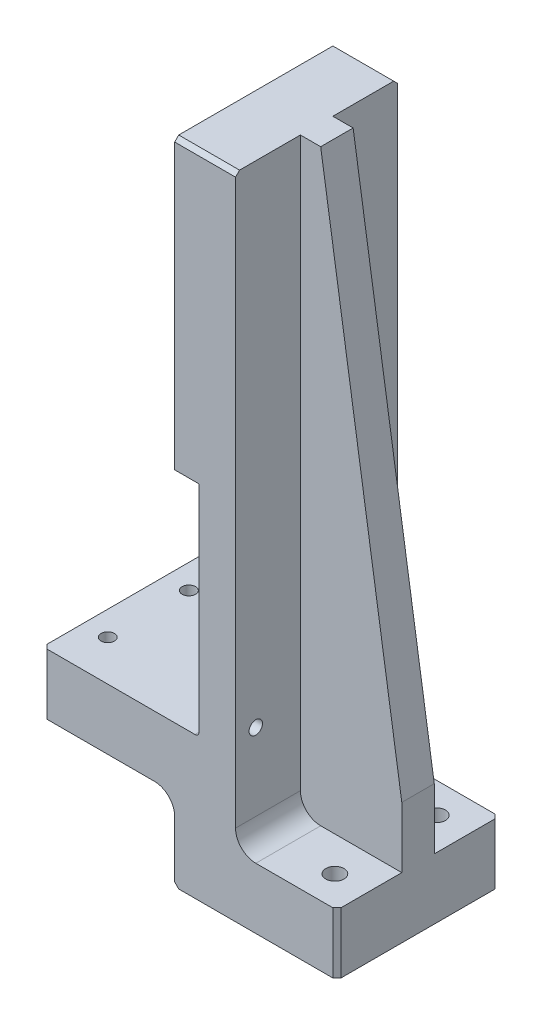
from build123d import *

# Parameters (mm, degrees)
BOSS_EXTRUDE1_DEPTH   = 20
BOSS_EXTRUDE2_DEPTH   = 4
SKETCH3_R             = 2.25
CUT_EXTRUDE2_DEPTH    = 164.343962239
M4_TAPPED_HOLE1_D     = 3.3
M4_TAPPED_HOLE2_D     = 3.3
M4_TAPPED_HOLE2_DEPTH = 11.5
M4_TAPPED_HOLE2_TIP   = 0.991420021
CUT_EXTRUDE3_REACH    = 151.937
SKETCH12_W            = 6
SKETCH12_H            = 54
M4_TAPPED_HOLE3_D     = 3.3
M4_TAPPED_HOLE3_DEPTH = 11.5
M4_TAPPED_HOLE3_TIP   = 0.991420021
CHAMFER1_SIZE         = 1
FILLET1_R             = 1
FILLET2_R             = 5


with BuildPart() as part:
    # Sketch1 → Boss-Extrude1 (new, symmetric)
    with BuildSketch(Plane.XY):
        Polygon((0, 0), (32.5, 0), (32.5, 125), (47.5, 125), (47.5, -20), (72.5, -20), (72.5, -35), (32.5, -35), (32.5, -15), (0, -15), align=None)
    extrude(amount=BOSS_EXTRUDE1_DEPTH, both=True)

    # Sketch2 → Boss-Extrude2 (add, symmetric)
    with BuildSketch(Plane.XY):
        Polygon((47.5, 125), (52.5, 125), (72.5, -5), (72.5, -20), (47.5, -20), align=None)
    extrude(amount=BOSS_EXTRUDE2_DEPTH, both=True)

    # Sketch3 → Cut-Extrude2 (cut, through all)
    with BuildSketch(Plane(origin=(0, -20, 0), x_dir=(1, 0, 0), z_dir=(0, 1, 0))):
        with Locations(Location((64.5, -12.5, 0), (0, 0, 270))):
            Circle(SKETCH3_R)
        with Locations(Location((64.5, 12.5, 0), (0, 0, 270))):
            Circle(SKETCH3_R)
    extrude(amount=-CUT_EXTRUDE2_DEPTH, mode=Mode.SUBTRACT)

    # M4 Tapped Hole1 (through all)
    with Locations(Plane(origin=(0, 0, 0), x_dir=(-1, 0, 0), z_dir=(0, 1, 0))):
        with Locations((-6, -10), (-6, 10)):
            Hole(M4_TAPPED_HOLE1_D / 2)

    # M4 Tapped Hole2
    with Locations(Plane(origin=(32.5, -167.050225356, 16.087508651), x_dir=(0, 0, 1), z_dir=(-1, 0, 0))):
        with Locations((-16.087508651, 276.050225356), (-16.087508651, 251.050225356)):
            Hole(M4_TAPPED_HOLE2_D / 2, depth=M4_TAPPED_HOLE2_DEPTH)
            with Locations((0, 0, -(M4_TAPPED_HOLE2_DEPTH + M4_TAPPED_HOLE2_TIP / 2))):  # 118° drill point
                Cone(0, M4_TAPPED_HOLE2_D / 2, M4_TAPPED_HOLE2_TIP, mode=Mode.SUBTRACT)

    # Sketch12 → Cut-Extrude3 (cut, up to next)
    with BuildSketch(Plane(origin=(0, 0, -20), x_dir=(-1, 0, 0), z_dir=(0, 0, -1)), mode=Mode.PRIVATE) as cut_extrude3_sk1:
        with Locations((-35.5, 27)):
            Rectangle(SKETCH12_W, SKETCH12_H)
    cut_extrude3_tool1 = extrude(cut_extrude3_sk1.sketch, amount=-CUT_EXTRUDE3_REACH, mode=Mode.PRIVATE) & part.part
    add(cut_extrude3_tool1.solids().sort_by_distance((35.5, 27, -20))[0], mode=Mode.SUBTRACT)

    # M4 Tapped Hole3
    with Locations(Plane.ZY.offset(-38.5)):
        with Locations((-15, 4), (15, 4)):
            Hole(M4_TAPPED_HOLE3_D / 2, depth=M4_TAPPED_HOLE3_DEPTH)
            with Locations((0, 0, -(M4_TAPPED_HOLE3_DEPTH + M4_TAPPED_HOLE3_TIP / 2))):  # 118° drill point
                Cone(0, M4_TAPPED_HOLE3_D / 2, M4_TAPPED_HOLE3_TIP, mode=Mode.SUBTRACT)

    # Chamfer1
    chamfer1_edges = [part.edges().sort_by_distance(p)[0] for p in [
        (40, 125, -20),
        (72.5, -27.5, -20),
        (0, -7.5, -20),
        (72.5, -27.5, 20),
        (32.5, -35, 0),
        (40, 125, 20),
        (0, -7.5, 20),
    ]]
    chamfer(chamfer1_edges, length=CHAMFER1_SIZE)

    # Fillet1
    fillet1_edges = [part.edges().sort_by_distance(p)[0] for p in [
        (38.5, 0, 0),
    ]]
    fillet(fillet1_edges, radius=FILLET1_R)

    # Fillet2
    fillet2_edges = [part.edges().sort_by_distance(p)[0] for p in [
        (47.5, -20, 12),
        (32.5, -15, 0),
        (47.5, -20, -12),
    ]]
    fillet(fillet2_edges, radius=FILLET2_R)


solid = part.part
